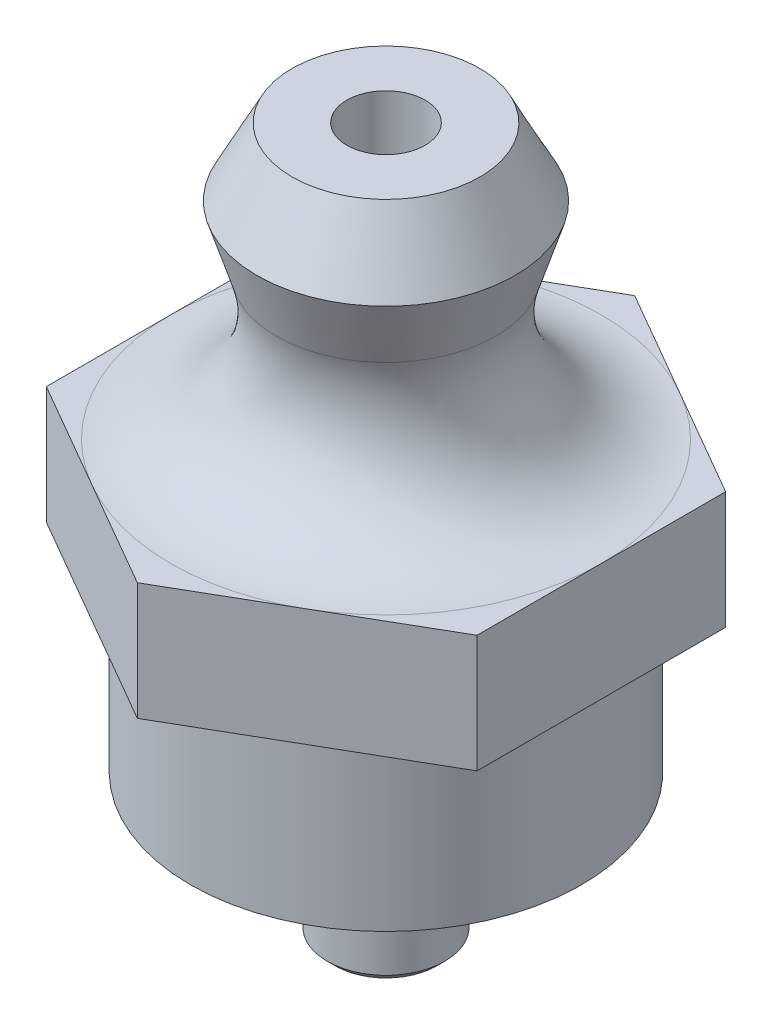
SolidWorks part; units mm, degrees
ref_plane "前视基准面" through (0, 0, 0) normal (0, 0, 1) x (1, 0, 0)
ref_plane "上视基准面" through (0, 0, 0) normal (0, 1, 0) x (1, 0, 0)
ref_plane "右视基准面" through (0, 0, 0) normal (1, 0, 0) x (0, 0, -1)
sketch "草图1" plane through (0, 0, 0) normal (0, 0, 1) x (1, 0, 0)
  line L0 (-1, 18) -> (-2.4, 18)
  line L1 (0, 0) -> (0, -3.114) construction
  line L2 (-2.4, 18) -> (-3.3, 16.2711)
  line L3 (-3.3, 16.2711) -> (-2.8, 14.6756)
  line L4 (0, 11) -> (-6.7881, 11) construction
  line L5 (0, 8) -> (-2.9677, 8) construction
  line L6 (-1, 0) -> (-1.5, 0)
  line L7 (-1.5, 0) -> (-1.5, 1.822)
  line L8 (-1.5, 1.822) -> (-5, 3.644)
  line L9 (-5, 3.644) -> (-5, 8)
  line L10 (-5, 8) -> (-5.5, 8)
  line L11 (-5.5, 8) -> (-5.5, 11)
  line L12 (-1, 0) -> (-1, 18)
  line L13 (-5, 3.644) -> (-5, 1.822) construction
  arc A0 (-5.5, 11) -> (-2.8, 14.6756) centre (-5.5, 13.8295) ccw
  dimension "D1" = 6.6
  dimension "hm" = 18
  dimension "d5" = 117.5
  dimension "D2" = 4.8
  dimension "h1" = 7
  dimension "h" = 10
  dimension "d" = 10
  dimension "sm" = 11
  dimension "D4" = 5.6
  dimension "D6" = 117.5
  dimension "D7" = 3
  dimension "D8" = 2
revolve "旋转2" add sketch "草图1" angle 360 about L1
cosmetic thread "装饰螺纹线1"
sketch "草图2" plane through (0, 8, 0) normal (0, -1, 0) x (1, 0, 0)
  line L1 (-5.5, 3.1754) -> (-5.5, -3.1754)
  line L2 (-5.5, -3.1754) -> (0, -6.3509)
  line L3 (0, -6.3509) -> (5.5, -3.1754)
  line L4 (5.5, -3.1754) -> (5.5, 3.1754)
  line L5 (5.5, 3.1754) -> (0, 6.3509)
  line L6 (0, 6.3509) -> (-5.5, 3.1754)
  circle A0 centre (0, 0) radius 5.5 construction
  circle A1 centre (0, 0) radius 5.5 construction
extrude "拉伸1" add sketch "草图2" against normal up to vertex (3 mm away) up to point (-5.5, 11, 0)
chamfer "倒角1" distance 0.2 angle 45 1 edges at (0, 0, 1.5)
